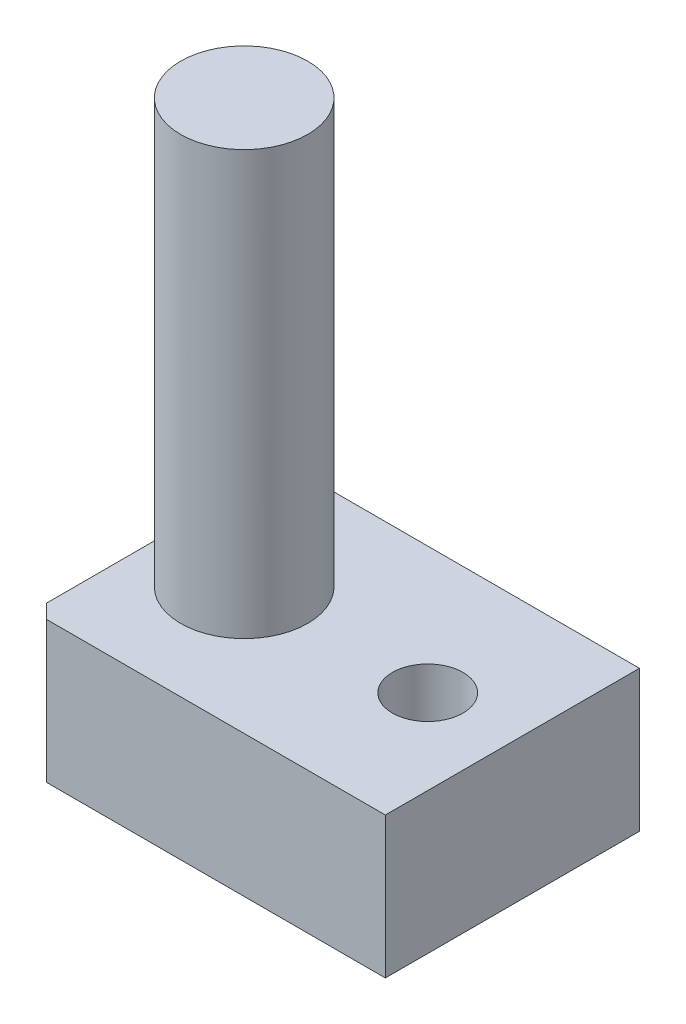
from build123d import *

# Parameters (mm, degrees)
SKETCH_1_W          = 25
SKETCH_1_H          = 10
EXTRUDE_1_DEPTH     = 18
SKETCH_2_R          = 4.5
EXTRUDE_2_DEPTH     = 30
CUT_EXTRUDE_1_REACH = 39.152
SKETCH_3_R          = 2.5
CHAMFER_1_SIZE      = 1


with BuildPart() as part:
    # 草图1 → 凸台-拉伸1 (new body)
    with BuildSketch(Plane.XY):
        Rectangle(SKETCH_1_W, SKETCH_1_H)
    extrude(amount=EXTRUDE_1_DEPTH)

    # 草图2 → 凸台-拉伸2 (add)
    with BuildSketch(Plane(origin=(0, 5, 0), x_dir=(1, 0, 0), z_dir=(0, 1, 0))):
        with Locations((-6.5, -9)):
            Circle(SKETCH_2_R)
    extrude(amount=EXTRUDE_2_DEPTH)

    # 草图3 → 切除-拉伸1 (cut, up to next)
    with BuildSketch(Plane(origin=(0, 5, 0), x_dir=(1, 0, 0), z_dir=(0, 1, 0)), mode=Mode.PRIVATE) as cut_extrude_1_sk1:
        with Locations(Location((6.5, -9, 0), (0, 0, 180))):
            Circle(SKETCH_3_R)
    cut_extrude_1_tool1 = extrude(cut_extrude_1_sk1.sketch, amount=-CUT_EXTRUDE_1_REACH, mode=Mode.PRIVATE) & part.part
    add(cut_extrude_1_tool1.solids().sort_by_distance((6.5, 5, 9))[0], mode=Mode.SUBTRACT)

    # 倒角1
    chamfer_1_edges = [part.edges().sort_by_distance(p)[0] for p in [
        (-12.5, 0, 18),
        (-12.5, 0, 0),
    ]]
    chamfer(chamfer_1_edges, length=CHAMFER_1_SIZE)


solid = part.part
